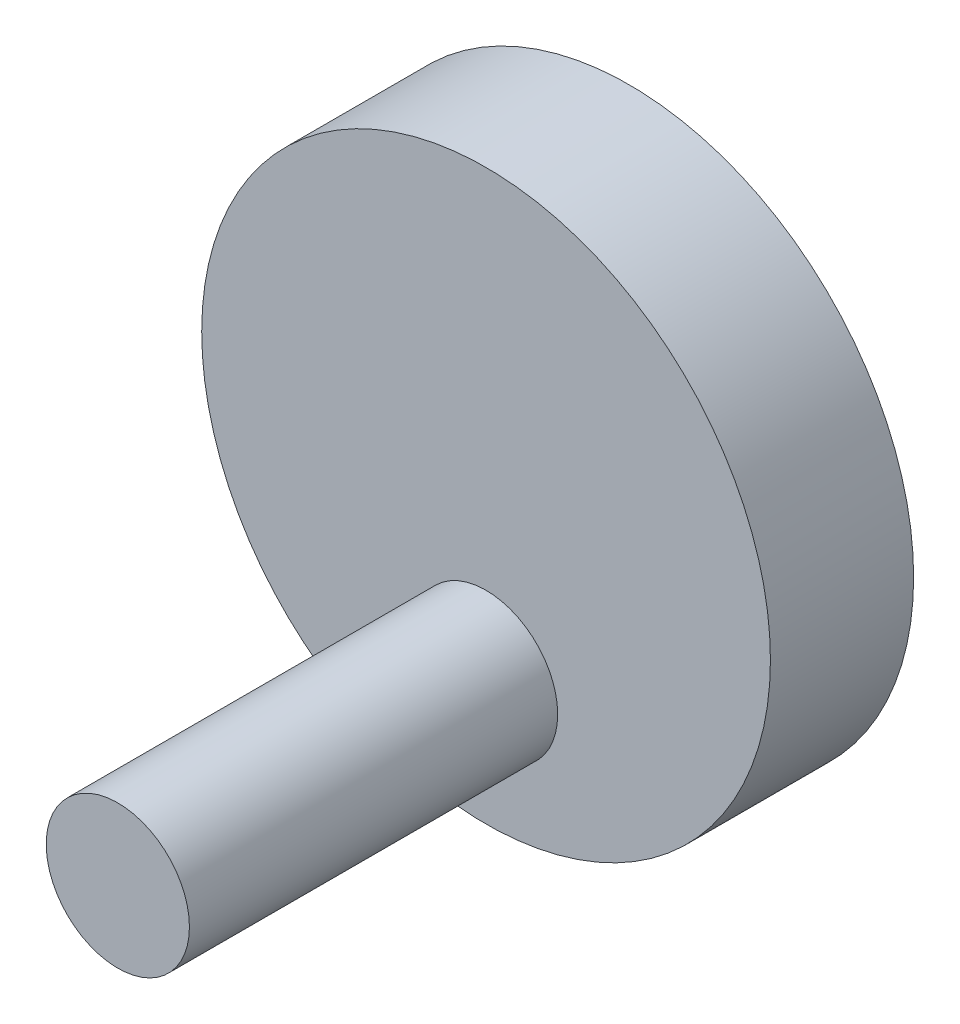
from build123d import *

# Parameters (mm, degrees)
BOSS_EXTRUDE1_DEPTH      = 2
BOSS_EXTRUDE1_DEPTH_BACK = 5
SKETCH1_R                = 13.9
SKETCH2_R                = 3.9
CUT_EXTRUDE1_DEPTH       = 6
SKETCH3_R                = 3.5
BOSS_EXTRUDE2_DEPTH      = 18


with BuildPart() as part:
    # Sketch1 → Boss-Extrude1 (new, two sides: drawn at the far end of the back side and taken through both)
    with BuildSketch(Plane.XY.offset(-BOSS_EXTRUDE1_DEPTH_BACK)):
        with Locations((0.613489308, -35)):
            Circle(SKETCH1_R)
    extrude(amount=BOSS_EXTRUDE1_DEPTH + BOSS_EXTRUDE1_DEPTH_BACK)

    # Sketch2 → Cut-Extrude1 (cut)
    with BuildSketch(Plane(origin=(0, 0, -5), x_dir=(-1, 0, 0), z_dir=(0, 0, -1))):
        with Locations((-0.613489308, -35)):
            Circle(SKETCH2_R)
    extrude(amount=-CUT_EXTRUDE1_DEPTH, mode=Mode.SUBTRACT)

    # Sketch3 → Boss-Extrude2 (add)
    with BuildSketch(Plane.XY.offset(2)):
        with Locations((0.613489308, -42.5)):
            Circle(SKETCH3_R)
    extrude(amount=BOSS_EXTRUDE2_DEPTH)


solid = part.part
